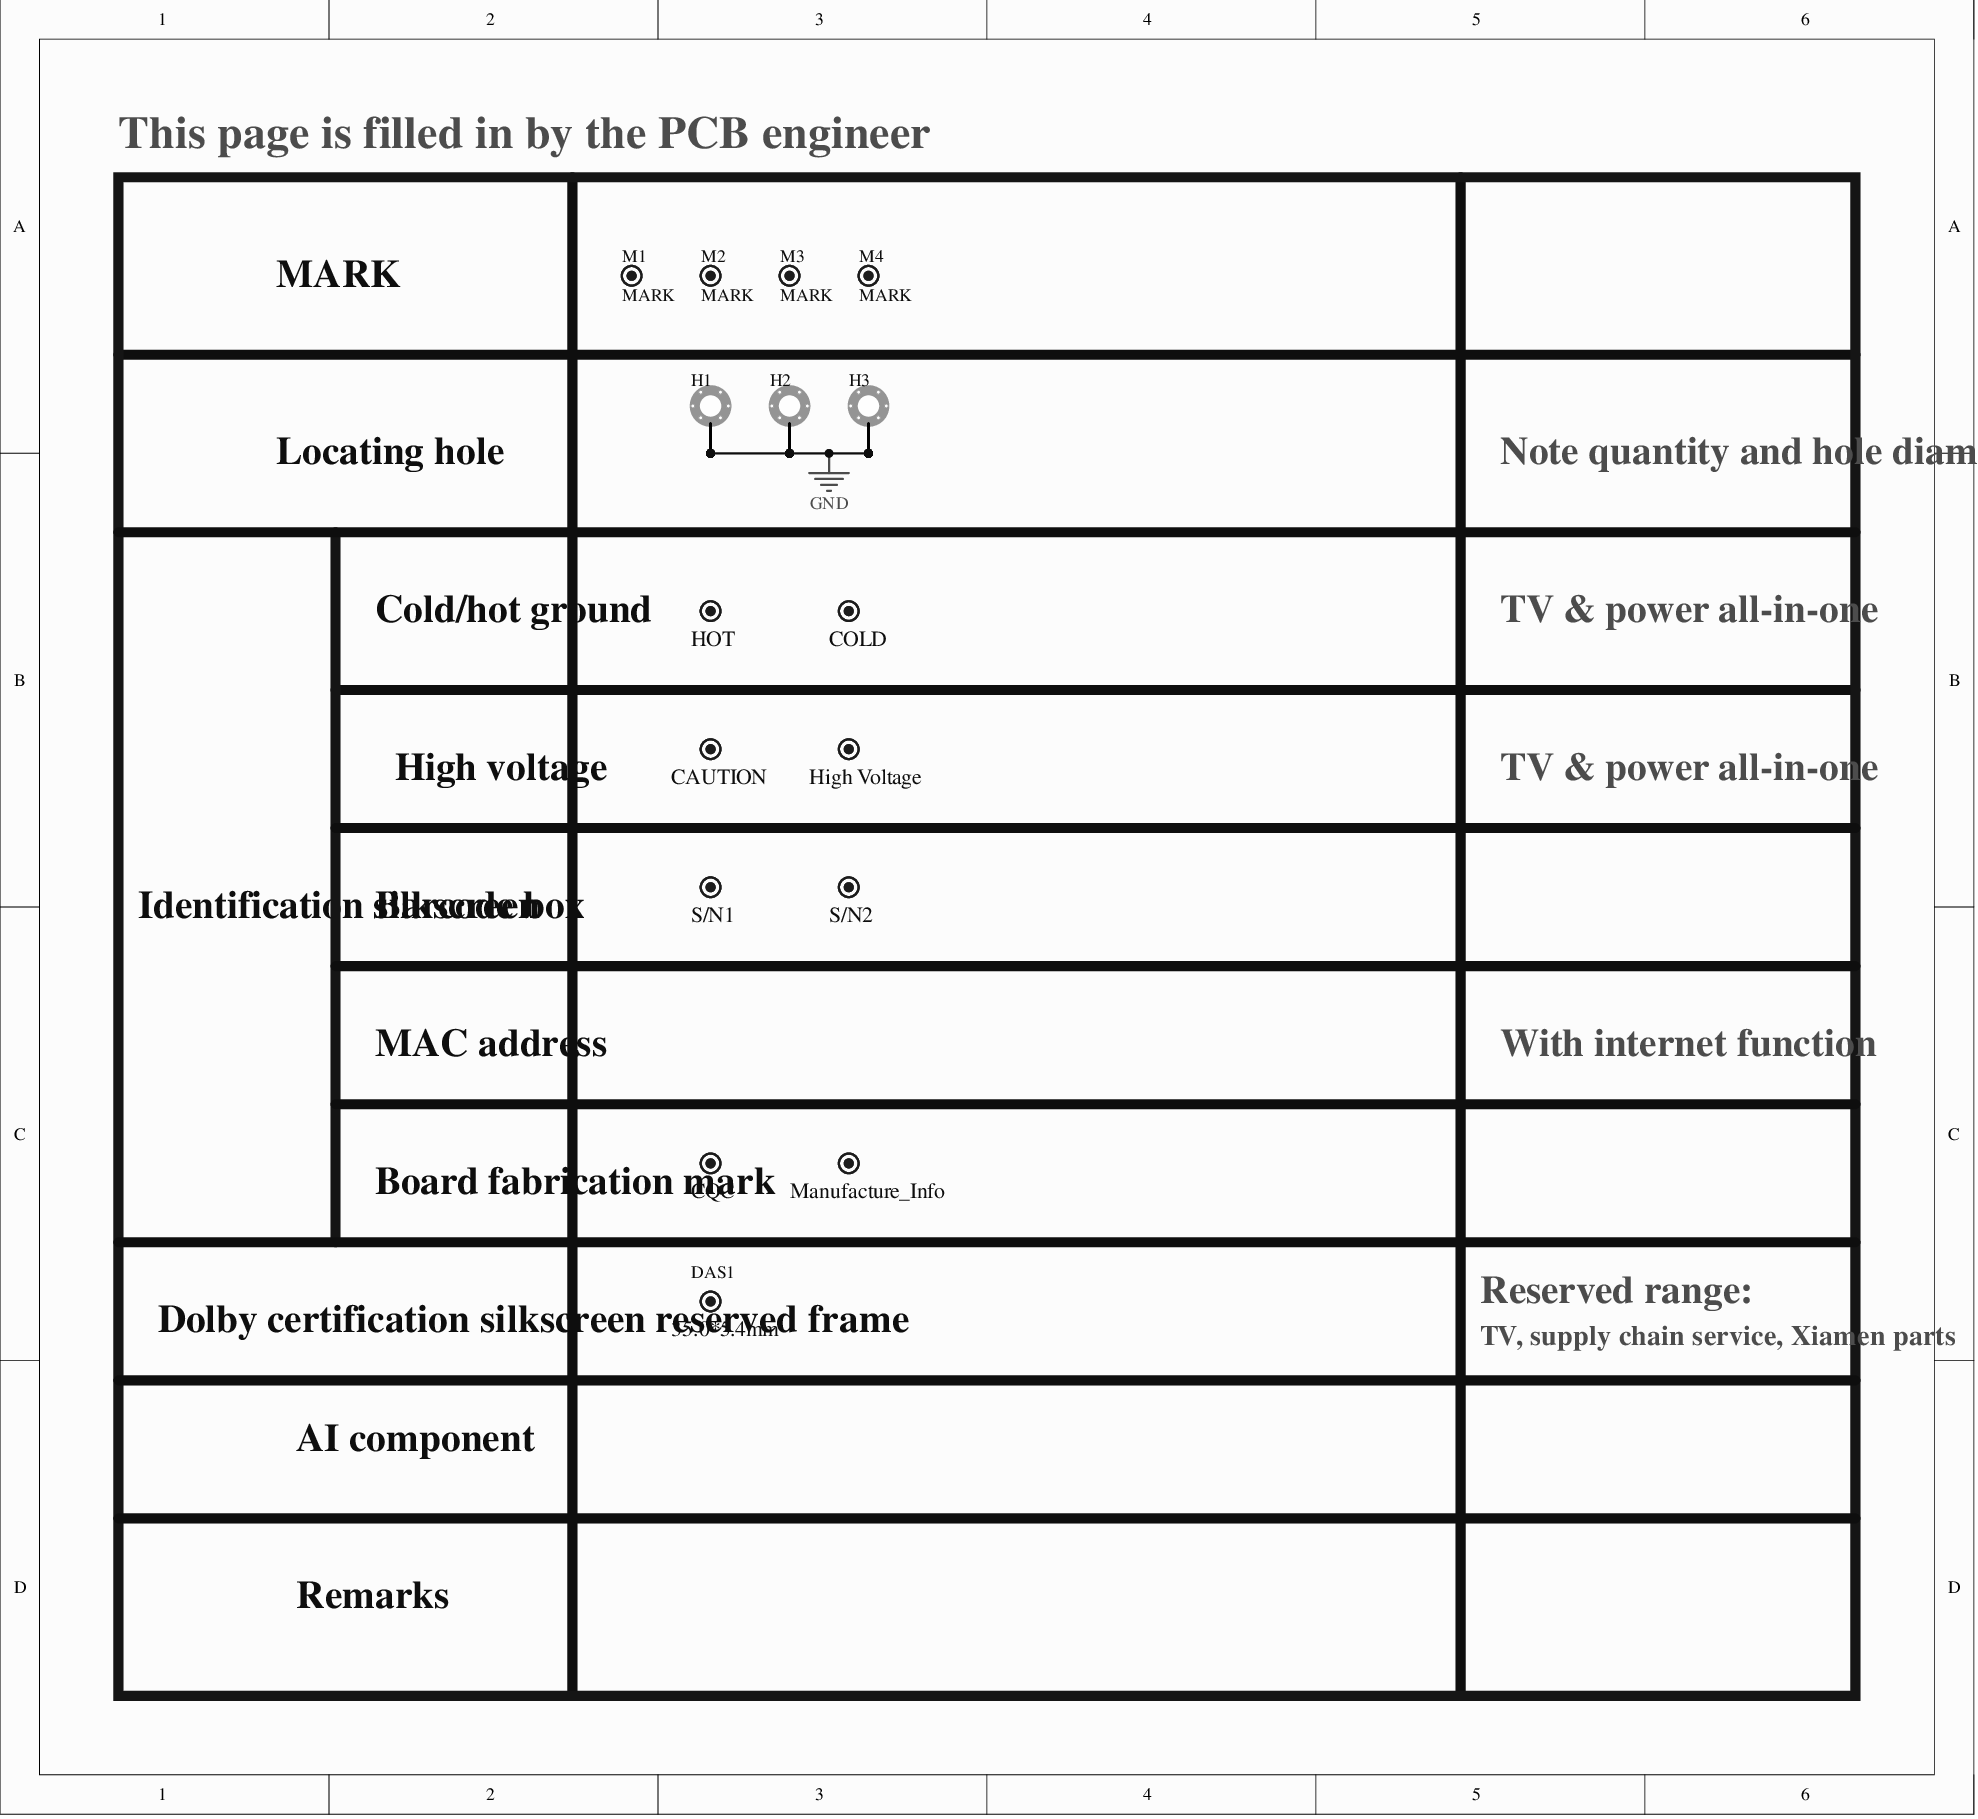
[diagram p0: MISC116569-3.SchDoc]
# Altium project MISC116569-15.PrjPCB (part 1 of 8)
12 sheets, 527 parts. Net scope: global (net labels, ports and power ports of the same name join across sheets).
Board file: MISC116569.PcbDoc
Sheets:
  MISC116569-3.SchDoc
  MISC116569-5.SchDoc
  MISC116569-14.SchDoc
  MISC116569-6.SchDoc
  MISC116569-7.SchDoc
  MISC116569-8.SchDoc
  MISC116569-9.SchDoc
  MISC116569-10.SchDoc
  MISC116569-11.SchDoc
  MISC116569-12.SchDoc
  MISC116569-13.SchDoc
  MISC116569-4.SchDoc

## Sheet MISC116569-3.SchDoc
size 254 x 233 mm

### Parts
CAUTION  CAUTION  [CAUTION]
COLD  COLD  [COLD]
CQC  CQC  [CQC]
DAS1  35.0*5.4mm  [DOLBY_AS2]
H1  Location hole  [ASSE4.0C-3]  (value not drawn)
H2  Location hole  [ASSE4.0C-3]  (value not drawn)
H3  Location hole  [ASSE4.0C-3]  (value not drawn)
High_Voltage  High Voltage  [High Voltage]
HOT  HOT  [HOT]
M1  MARK  [MARK]
M2  MARK  [MARK]
M3  MARK  [MARK]
M4  MARK  [MARK]
Manufacture_Info  Manufacture_Info  [Manufacture_Info]
S/N1  Barcode  [Barcode]  (value not drawn)
S/N2  Barcode  [Barcode]  (value not drawn)

### Nets
GND: H1.1 H1.2 H1.3 H1.4 H1.5 H1.6 H2.1 H2.2 H2.3 H2.4 H2.5 H2.6 H3.1 H3.2 H3.3 H3.4 H3.5 H3.6

### Notes on the sheet
- This page is filled in by the PCB engineer
- MARK
- Locating hole
- Note quantity and hole diameter
- (near HOT) Cold/hot ground
- TV & power all-in-one
- High voltage
- Identification silkscreen
- Barcode box
- MAC address
- With internet function
- (near CQC) Board fabrication mark
- (near DAS1) Dolby certification silkscreen reserved frame
- Reserved range:
- TV, supply chain service, Xiamen parts
- AI component
- Remarks

### Library data of the parts
DAS1 = DOLBY_AS2
H1-H3 = Location hole-D
M1-M4 = MARK-D

## Sheet MISC116569-5.SchDoc
size 254 x 322 mm
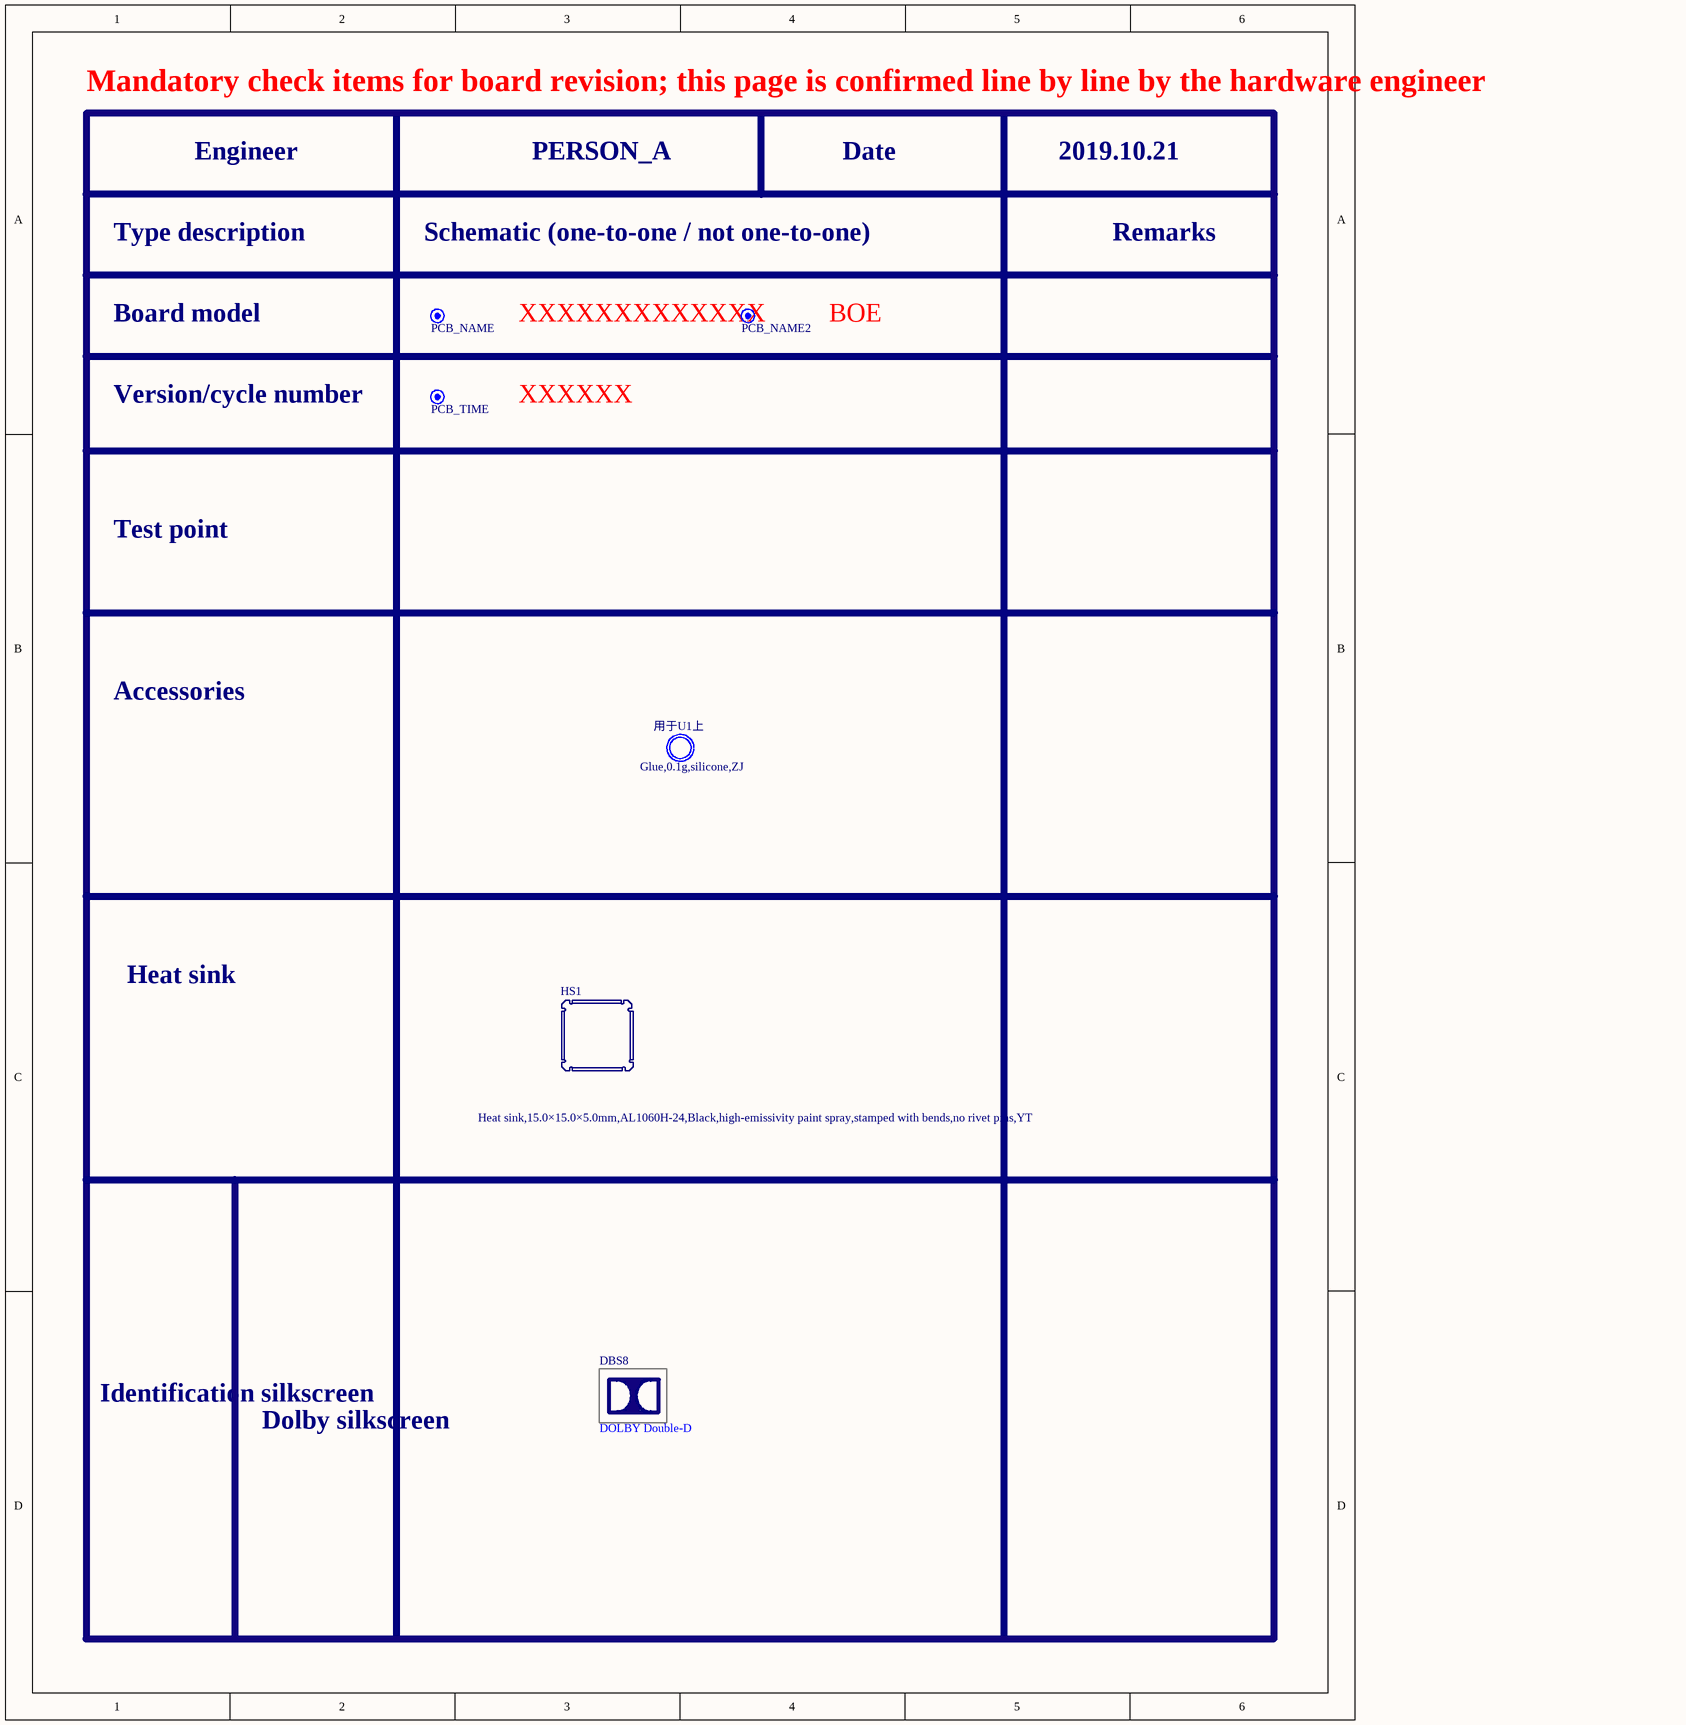
[diagram p1: MISC116569-5.SchDoc]

### Parts
BOE  PCB_NAME2  [PCB_NAME]
DBS8  DOLBY Double-D  [Double-D-SILK]
HS1  Heat sink,15.0×15.0×5.0mm,AL1060H-24,Black,high-emissivity paint spray,stamped with bends,no rivet pins,YT  [HS(15X15X5)-S]
XXXXXX  PCB_TIME  [PCB_TIME]
XXXXXXXXXXXXX  PCB_NAME  [PCB_NAME]
用于U1上  Glue,0.1g,silicone,ZJ  [Heat-Shrinkable Tube]

### Notes on the sheet
- Mandatory check items for board revision; this page is confirmed line by line by the hardware engineer
- Engineer
- PERSON_A
- Date
- 2019.10.21
- Type description
- Schematic (one-to-one / not one-to-one)
- Remarks
- Board model
- Version/cycle number
- Test point
- Accessories
- Heat sink
- Identification silkscreen
- Dolby silkscreen

### Library data of the parts
BOE = PCB_NAME
HS1 = 004.040.0008928-D: Heat sink,15.0×15.0×5.0mm,AL1060H-24,Black,high-emissivity paint spray,stamped with bends,no rivet pins,YT-D
用于U1上 = Φ12mm×12mm-黑色-125度(UL认证)-D